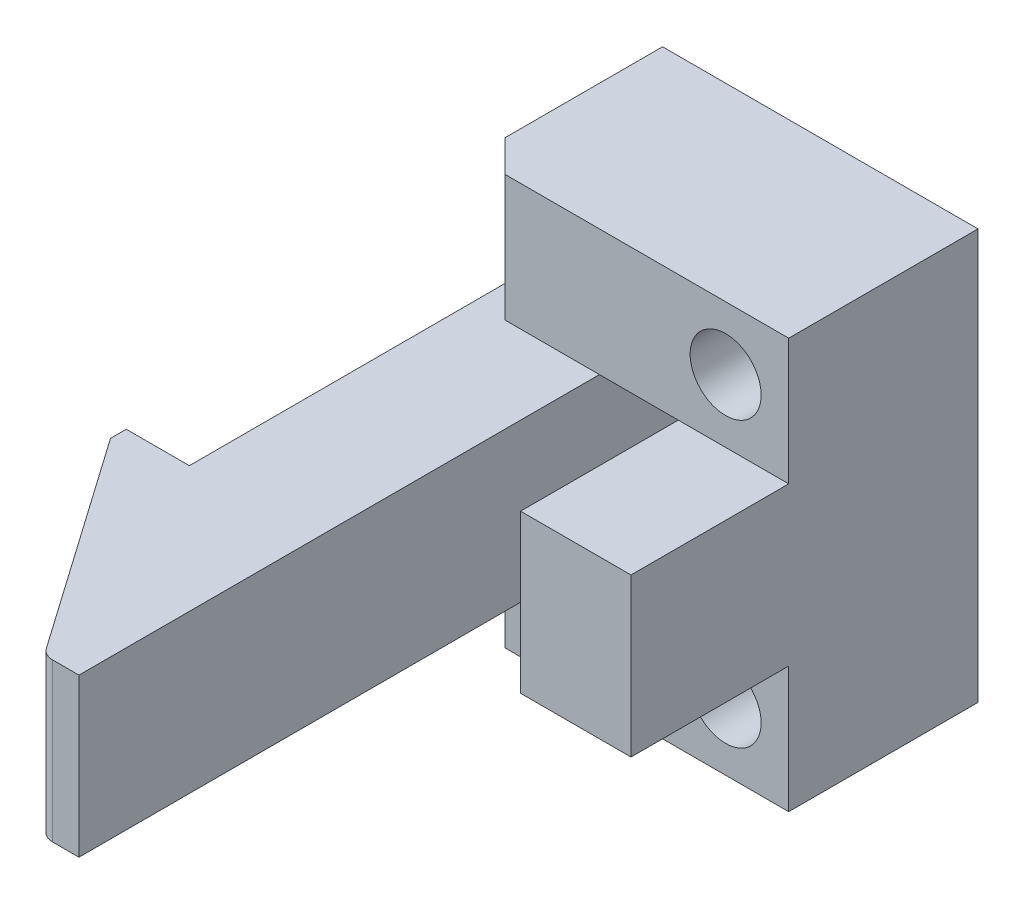
from build123d import *

# Parameters (mm, degrees)
SKETCH1_W                = 20
SKETCH1_H                = 26
BOSS_EXTRUDE1_DEPTH      = 12
CUT_EXTRUDE1_REACH       = 22.322
SKETCH2_R                = 2.25
SKETCH3_W                = 7
SKETCH3_H                = 10
BOSS_EXTRUDE2_DEPTH      = 10
CUT_EXTRUDE2_REACH       = 22.322
SKETCH4_W                = 13
SKETCH4_H                = 10
BOSS_EXTRUDE3_DEPTH      = 5
BOSS_EXTRUDE3_DEPTH_BACK = 5
CHAMFER1_SIZE            = 2
FILLET1_R                = 1


with BuildPart() as part:
    # Sketch1 → Boss-Extrude1 (new body)
    with BuildSketch(Plane.XY):
        Rectangle(SKETCH1_W, SKETCH1_H)
    extrude(amount=BOSS_EXTRUDE1_DEPTH)

    # Sketch2 → Cut-Extrude1 (cut, up to next)
    with BuildSketch(Plane.XY.offset(12), mode=Mode.PRIVATE) as cut_extrude1_sk1:
        with Locations((6, 9)):
            Circle(SKETCH2_R)
    cut_extrude1_tool1 = extrude(cut_extrude1_sk1.sketch, amount=-CUT_EXTRUDE1_REACH, mode=Mode.PRIVATE) & part.part
    # Sketch2 → Cut-Extrude1 (cut, up to next)
    with BuildSketch(Plane.XY.offset(12), mode=Mode.PRIVATE) as cut_extrude1_sk2:
        with Locations((6, -9)):
            Circle(SKETCH2_R)
    cut_extrude1_tool2 = extrude(cut_extrude1_sk2.sketch, amount=-CUT_EXTRUDE1_REACH, mode=Mode.PRIVATE) & part.part
    add(cut_extrude1_tool1.solids().sort_by_distance((6, 9, 12))[0], mode=Mode.SUBTRACT)
    add(cut_extrude1_tool2.solids().sort_by_distance((6, -9, 12))[0], mode=Mode.SUBTRACT)

    # Sketch3 → Boss-Extrude2 (add)
    with BuildSketch(Plane.XY.offset(12)):
        with Locations((6.5, 0)):
            Rectangle(SKETCH3_W, SKETCH3_H)
    extrude(amount=BOSS_EXTRUDE2_DEPTH)

    # Sketch4 → Cut-Extrude2 (cut, up to next)
    with BuildSketch(Plane.XY.offset(12), mode=Mode.PRIVATE) as cut_extrude2_sk1:
        with Locations((-3.5, 0)):
            Rectangle(SKETCH4_W, SKETCH4_H)
    cut_extrude2_tool1 = extrude(cut_extrude2_sk1.sketch, amount=-CUT_EXTRUDE2_REACH, mode=Mode.PRIVATE) & part.part
    add(cut_extrude2_tool1.solids().sort_by_distance((-3.5, 0, 12))[0], mode=Mode.SUBTRACT)

    # Chamfer1
    chamfer1_edges = [part.edges().sort_by_distance(p)[0] for p in [
        (-10, -9, 12),
        (-10, 9, 12),
    ]]
    chamfer(chamfer1_edges, length=CHAMFER1_SIZE)


with BuildPart() as body_2:
    # Sketch5 → Boss-Extrude3 (new, two sides: drawn at the far end of the back side and taken through both)
    with BuildSketch(Plane(origin=(0, 0, 0), x_dir=(1, 0, 0), z_dir=(0, 1, 0)).offset(-BOSS_EXTRUDE3_DEPTH_BACK)):
        Polygon((-10, -2), (-10, -30), (-14, -30), (-14, -31), (-4.197094465, -45), (-2, -45), (-2, -2), align=None)
    extrude(amount=BOSS_EXTRUDE3_DEPTH + BOSS_EXTRUDE3_DEPTH_BACK)

    # Fillet1
    fillet1_edges = [body_2.edges().sort_by_distance(p)[0] for p in [
        (-4.197094465, 0, 45),
    ]]
    fillet(fillet1_edges, radius=FILLET1_R)


solid = Compound([part.part, body_2.part])
